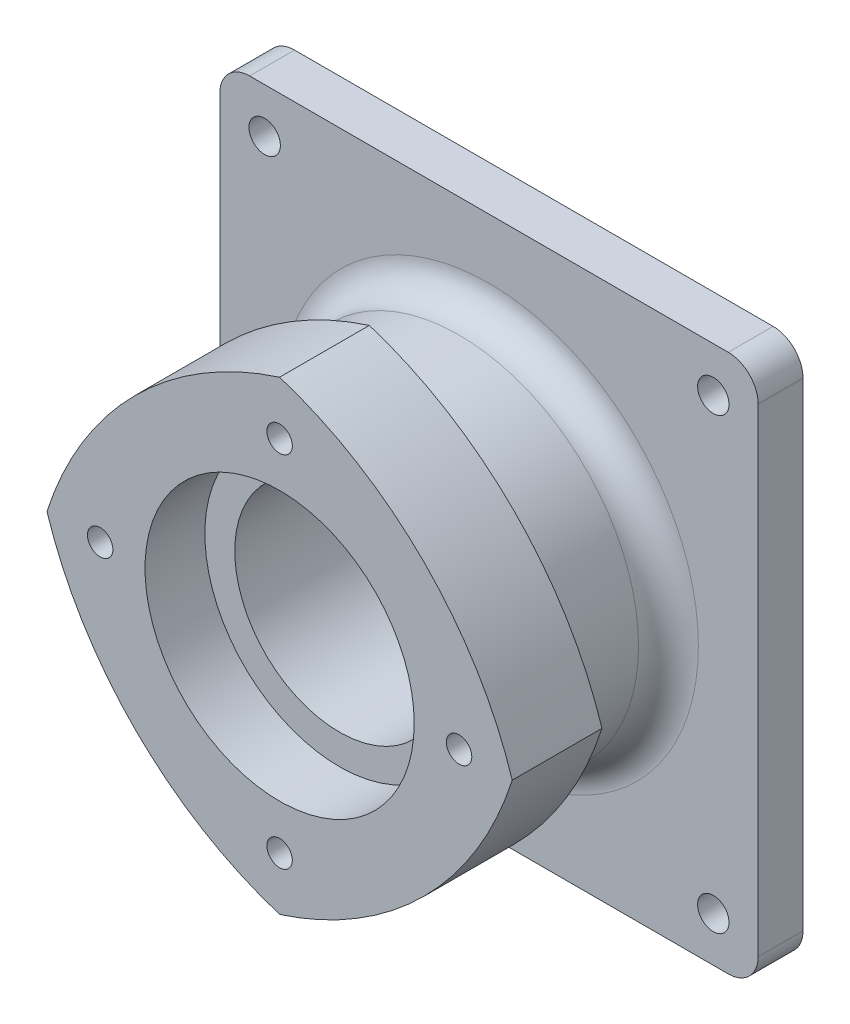
from build123d import *

# Parameters (mm, degrees)
SKETCH_1_R               = 5.25
EXTRUDE_1_DEPTH          = 15
SKETCH_2_R               = 60
EXTRUDE_2_DEPTH          = 40
EXTRUDE_3_DEPTH          = 30
PATTERN_CIRCULAR_1_COUNT = 4
FILLET_1_R               = 10
FILLET_2_R               = 5
SKETCH_6_R               = 35
CUT_EXTRUDE_1_DEPTH      = 154.05227865
SKETCH_7_R               = 45
CUT_EXTRUDE_2_DEPTH      = 20


with BuildPart() as part:
    # 草图1 → 凸台-拉伸1 (new body)
    with BuildSketch(Plane.XY):
        with BuildLine():
            Line((-80, 90), (80, 90))
            ThreePointArc((80, 90), (87.071067812, 87.071067812), (90, 80))
            Line((90, 80), (90, -80))
            ThreePointArc((90, -80), (87.071067812, -87.071067812), (80, -90))
            Line((80, -90), (-80, -90))
            ThreePointArc((-80, -90), (-87.071067812, -87.071067812), (-90, -80))
            Line((-90, -80), (-90, 80))
            ThreePointArc((-90, 80), (-87.071067812, 87.071067812), (-80, 90))
        make_face()
        with Locations((-75, 75)):
            Circle(SKETCH_1_R, mode=Mode.SUBTRACT)
        with Locations((75, 75)):
            Circle(SKETCH_1_R, mode=Mode.SUBTRACT)
        with Locations((-75, -75)):
            Circle(SKETCH_1_R, mode=Mode.SUBTRACT)
        with Locations((75, -75)):
            Circle(SKETCH_1_R, mode=Mode.SUBTRACT)
    extrude(amount=EXTRUDE_1_DEPTH)

    # 草图2 → 凸台-拉伸2 (add)
    with BuildSketch(Plane.XY.offset(15)):
        Circle(SKETCH_2_R)
    extrude(amount=EXTRUDE_2_DEPTH)

    # 草图3 → 凸台-拉伸3 (add)
    with BuildSketch(Plane.XY.offset(55)):
        with BuildLine():
            ThreePointArc((0, 77.781745931), (48.328171063, 48.328171063), (77.781745931, 0))
            ThreePointArc((77.781745931, 0), (48.328171063, -48.328171063), (0, -77.781745931))
            ThreePointArc((0, -77.781745931), (-48.328171063, -48.328171063), (-77.781745931, 0))
            ThreePointArc((-77.781745931, 0), (-48.328171063, 48.328171063), (0, 77.781745931))
        make_face()
    extrude(amount=EXTRUDE_3_DEPTH)

    # 草图5 → M10 螺纹孔1 (revolve, cut)
    with BuildSketch(Plane(origin=(0, 60, 85), x_dir=(0, -1, 0), z_dir=(1, 0, 0))):
        Polygon((0, 0), (0, 24.553657631), (4.25, 22), (4.25, 0), align=None)
    hole_wizard_m10_1 = revolve(axis=Axis((0, 60, 91.35), (0, 0, -1)), mode=Mode.SUBTRACT)

    # 阵列(圆周)1: M10 螺纹孔1 ×4 about axis
    pattern_circular_1_axis = Axis((0, 0, 0), (0, 0, 1))
    for i in range(1, PATTERN_CIRCULAR_1_COUNT):
        add(hole_wizard_m10_1.rotate(pattern_circular_1_axis, i * 360 / PATTERN_CIRCULAR_1_COUNT), mode=Mode.SUBTRACT)

    # 圆角1
    fillet_1_edges = [part.edges().sort_by_distance(p)[0] for p in [
        (-60, 0, 15),
    ]]
    fillet(fillet_1_edges, radius=FILLET_1_R)

    # 圆角2
    fillet_2_edges = [part.edges().sort_by_distance(p)[0] for p in [
        (-60, 0, 55),
    ]]
    fillet(fillet_2_edges, radius=FILLET_2_R)

    # 草图6 → 切除-拉伸1 (cut, through all)
    with BuildSketch(Plane.XY.offset(85)):
        Circle(SKETCH_6_R)
    extrude(amount=-CUT_EXTRUDE_1_DEPTH, mode=Mode.SUBTRACT)

    # 草图7 → 切除-拉伸2 (cut)
    with BuildSketch(Plane.XY.offset(85)):
        Circle(SKETCH_7_R)
    extrude(amount=-CUT_EXTRUDE_2_DEPTH, mode=Mode.SUBTRACT)


solid = part.part
